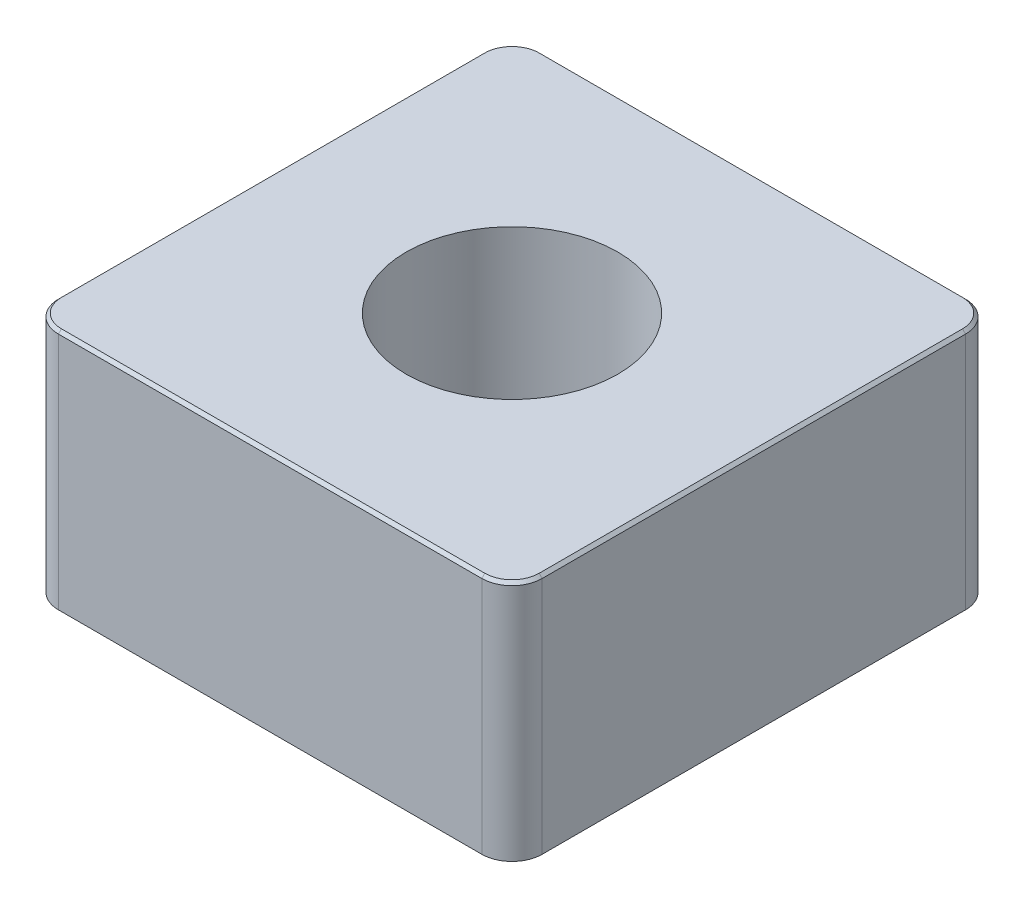
SolidWorks part; units mm, degrees
ref_plane "Front Plane" through (0, 0, 0) normal (0, 0, 1) x (1, 0, 0)
ref_plane "Top Plane" through (0, 0, 0) normal (0, 1, 0) x (1, 0, 0)
ref_plane "Right Plane" through (0, 0, 0) normal (1, 0, 0) x (0, 0, -1)
ref_plane "Plane4" through (0, 15, 0) normal (0, 1, 0) x (1, 0, 0)
sketch "Sketch1" plane through (0, 15, 0) normal (0, 1, 0) x (1, 0, 0)
  line L0 (-40, -40) -> (40, -40)
  line L1 (40, -40) -> (40, 40)
  line L2 (40, 40) -> (-40, 40)
  line L3 (-40, 40) -> (-40, -40)
  dimension "D1" = 80
extrude "Boss-Extrude1" add sketch "Sketch1" against normal blind 40
hole_wizard "M30 Clearance Hole1" positions "Sketch3" profile "Sketch2" hole size "M30" standard "ANSI Metric" end condition through all
sketch "Sketch3" plane through (0, 15, 0) normal (0, 1, 0) x (1, 0, 0)
  point P0 (0, 0)
sketch "Sketch2" plane through (0, 15, 0) normal (1, 0, 0) x (0, 0, 1)
  line L0 (0, 0) -> (0, 40)
  line L1 (0, 40) -> (17.5, 40)
  line L2 (17.5, 40) -> (17.5, 0)
  line L5 (17.5, 0) -> (0, 0)
  line L11 (0, -6.35) -> (0, 107.95) construction
  dimension "通孔孔直径" = 35
  dimension "通孔孔深度" = 40
fillet "Fillet1" radius 5 4 edges at (40, -5, 40) (-40, -5, 40) (40, -5, -40) (-40, -5, -40)
chamfer "Chamfer1" distance 0.5 angle 45 8 edges at (0, 15, -40) (-38.5355, 15, -38.5355) (38.5355, 15, -38.5355) (-40, 15, 0) (40, 15, 0) (-38.5355, 15, 38.5355) (38.5355, 15, 38.5355) (0, 15, 40)
